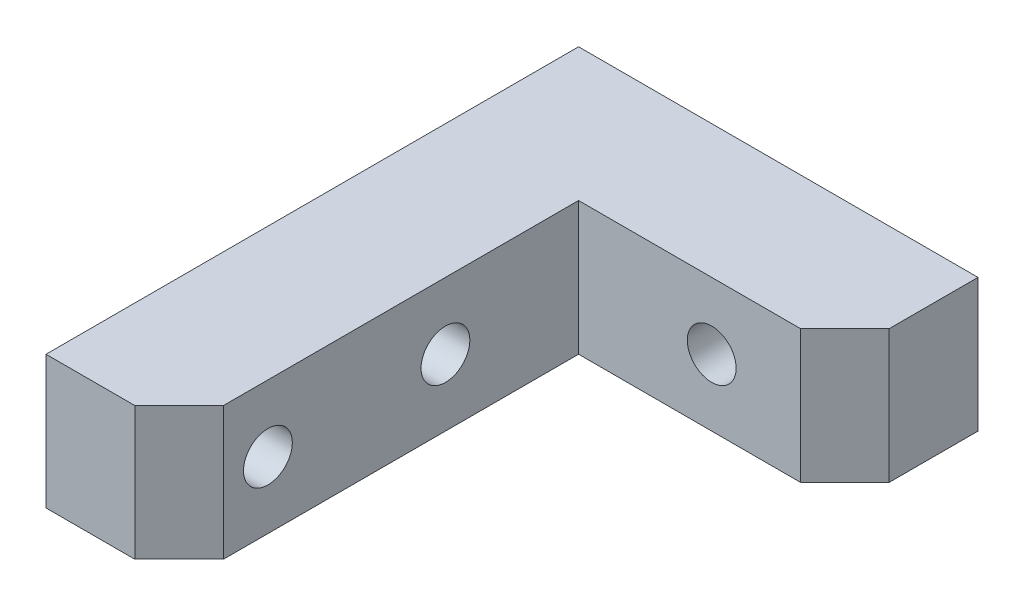
SolidWorks part; units mm, degrees
material "6061"
ref_plane "前视基准面" through (0, 0, 0) normal (0, 0, 1) x (1, 0, 0)
ref_plane "上视基准面" through (0, 0, 0) normal (0, 1, 0) x (1, 0, 0)
ref_plane "右视基准面" through (0, 0, 0) normal (1, 0, 0) x (0, 0, -1)
sketch "草图1" plane through (0, 0, 0) normal (0, 1, 0) x (1, 0, 0)
  line L0 (30, 0) -> (0, 0)
  line L1 (30, 15) -> (-15, 15)
  line L2 (30, 15) -> (30, 0)
  line L3 (0, -45) -> (-15, -45)
  line L4 (-15, 15) -> (-15, -45)
  line L7 (0, 0) -> (0, -45)
  point P0 (0, 0)
  dimension "D1" = 45
  dimension "D2" = 60
  dimension "D3" = 15
  dimension "D4" = 15
extrude "凸台-拉伸1" add sketch "草图1" along normal mid plane 15
chamfer "倒角1" distance 5 angle 45 2 edges at (0, 0, 45) (30, 0, 0)
hole_wizard "Ø5.5 (5.5) 直径孔1" positions "草图2" profile "草图3" hole size "Ø5.5" standard "ISO" end condition through all
sketch "草图2" plane through (0, 0, 0) normal (1, 0, 0) x (0, 0, -1)
  line L0 (0, 0) -> (-40.2625, 0) construction
  line L2 (-45, -7.5) -> (-45, 7.5) construction
  point P0 (-35, 0)
  point P2 (-15, 0)
  dimension "D1" = 10
  dimension "D2" = 20
sketch "草图3" plane through (0, 0, 35) normal (0, 1, 0) x (0, 0, -1)
  line L0 (0, 0) -> (0, 15)
  line L1 (0, 15) -> (2.75, 15)
  line L2 (2.75, 15) -> (2.75, 0)
  line L5 (2.75, 0) -> (0, 0)
  line L11 (0, -6.35) -> (0, 107.95) construction
  dimension "通孔孔直径" = 5.5
  dimension "通孔孔深度" = 15
hole_wizard "Ø5.5 (5.5) 直径孔2" positions "草图4" profile "草图5" hole size "Ø5.5" standard "ISO" end condition through all
sketch "草图4" plane through (0, 0, 0) normal (0, 0, 1) x (1, 0, 0)
  line L0 (0, 0) -> (25.8471, 0) construction
  line L2 (0, 7.5) -> (0, -7.5) construction
  point P0 (15, 0)
  dimension "D1" = 15
sketch "草图5" plane through (15, 0, 0) normal (1, 0, 0) x (0, -1, 0)
  line L0 (0, 0) -> (0, 15)
  line L1 (0, 15) -> (2.75, 15)
  line L2 (2.75, 15) -> (2.75, 0)
  line L5 (2.75, 0) -> (0, 0)
  line L11 (0, -6.35) -> (0, 107.95) construction
  dimension "通孔孔直径" = 5.5
  dimension "通孔孔深度" = 15
